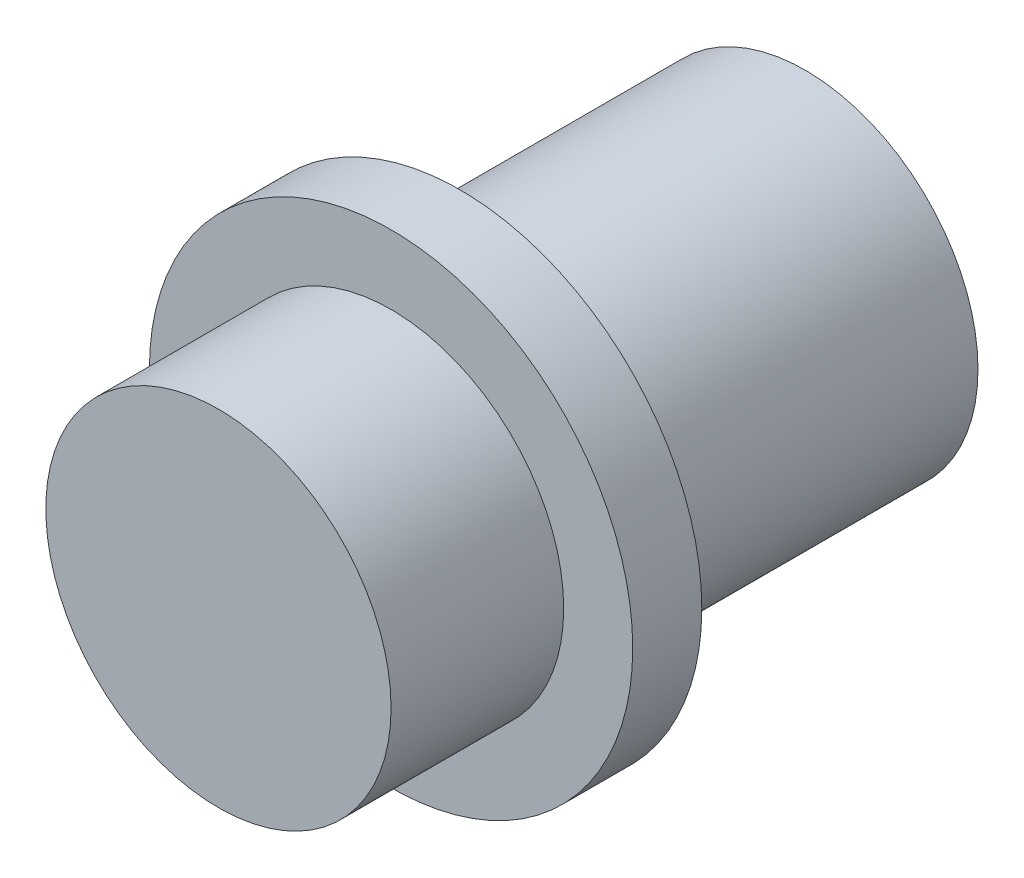
SolidWorks part; units mm, degrees
ref_plane "Front Plane" through (0, 0, 0) normal (0, 0, 1) x (1, 0, 0)
ref_plane "Top Plane" through (0, 0, 0) normal (0, 1, 0) x (1, 0, 0)
ref_plane "Right Plane" through (0, 0, 0) normal (1, 0, 0) x (0, 0, -1)
sketch "Sketch1" plane through (0, 0, 0) normal (0, 0, 1) x (1, 0, 0)
  circle A0 centre (0, 0) radius 5
  dimension "D1" = 10
extrude "Boss-Extrude1" add sketch "Sketch1" along normal blind 10
sketch "Sketch2" plane through (0, 0, 10) normal (0, 0, 1) x (1, 0, 0)
  circle A0 centre (0, 0) radius 7
  dimension "D1" = 14
extrude "Boss-Extrude2" add sketch "Sketch2" along normal blind 2
sketch "Sketch4" plane through (0, 0, 12) normal (0, 0, 1) x (1, 0, 0)
  circle A0 centre (0, 0) radius 5
  dimension "D1" = 10
extrude "Boss-Extrude3" add sketch "Sketch4" along normal blind 5
